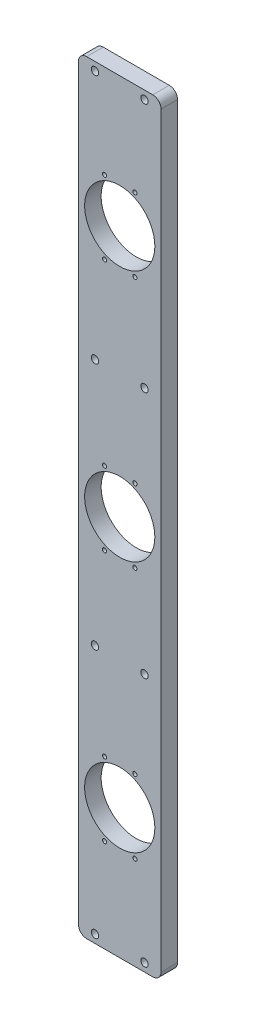
from build123d import *

# Parameters (mm, degrees)
SKETCH_1_W                   = 100
SKETCH_1_H                   = 925
EXTRUDE_1_DEPTH              = 20
HOLE_WIZARD_M6_2_D           = 5
SKETCH_11_R                  = 42.5
CUT_EXTRUDE_1_DEPTH          = 466.624580537
HOLE_WIZARD_M8_2_D           = 9
HOLE_WIZARD_M8_2_CBORE_D     = 15
HOLE_WIZARD_M8_2_CBORE_DEPTH = 8.6
FILLET_2_R                   = 10
SKETCH_14_R                  = 42.5
CUT_EXTRUDE_2_DEPTH          = 466.624580537
HOLE_WIZARD_M6_3_D           = 5


with BuildPart() as part:
    # 草图1 → 凸台-拉伸1 (new body)
    with BuildSketch(Plane.XY):
        Rectangle(SKETCH_1_W, SKETCH_1_H)
    extrude(amount=EXTRUDE_1_DEPTH)

    # M6 螺纹孔2 (through all)
    with Locations(Plane.XY.offset(20)):
        with Locations((-18.368804754, -260.653782439), (18.368804754, -260.653782439), (18.368804754, -349.346217561), (-18.368804754, -349.346217561), (18.368804754, 349.346217561), (-18.368804754, 349.346217561), (18.368804754, 260.653782439), (-18.368804754, 260.653782439)):
            Hole(HOLE_WIZARD_M6_2_D / 2)

    # 草图11 → 切除-拉伸1 (cut, through all)
    with BuildSketch(Plane.XY.offset(20)):
        with Locations((0, -305)):
            Circle(SKETCH_11_R)
    cut_extrude_1 = extrude(amount=-CUT_EXTRUDE_1_DEPTH, mode=Mode.SUBTRACT)

    # M8 六角凹头螺钉的柱形沉头孔2 (through all)
    with Locations(Plane(origin=(0, 0, 0), x_dir=(-1, 0, 0), z_dir=(0, 0, -1))):
        with Locations((-30, -452.5), (30, -452.5), (-30, -150), (30, -150), (30, 150), (-30, 150), (30, 452.5), (-30, 452.5)):
            CounterBoreHole(HOLE_WIZARD_M8_2_D / 2, HOLE_WIZARD_M8_2_CBORE_D / 2, HOLE_WIZARD_M8_2_CBORE_DEPTH)

    # 镜向10: 切除-拉伸1 across plane
    add(cut_extrude_1.mirror(Plane.ZX), mode=Mode.SUBTRACT)

    # 圆角2
    fillet_2_edges = [part.edges().sort_by_distance(p)[0] for p in [
        (50, -462.5, 10),
        (-50, -462.5, 10),
        (-50, 462.5, 10),
        (50, 462.5, 10),
    ]]
    fillet(fillet_2_edges, radius=FILLET_2_R)

    # 草图14 → 切除-拉伸2 (cut, through all)
    with BuildSketch(Plane.XY.offset(20)):
        Circle(SKETCH_14_R)
    extrude(amount=-CUT_EXTRUDE_2_DEPTH, mode=Mode.SUBTRACT)

    # M6 螺纹孔3 (through all)
    with Locations(Plane.XY.offset(20)):
        with Locations((-18.368804754, 44.346217561), (18.368804754, 44.346217561), (18.368804754, -44.346217561), (-18.368804754, -44.346217561)):
            Hole(HOLE_WIZARD_M6_3_D / 2)


solid = part.part
